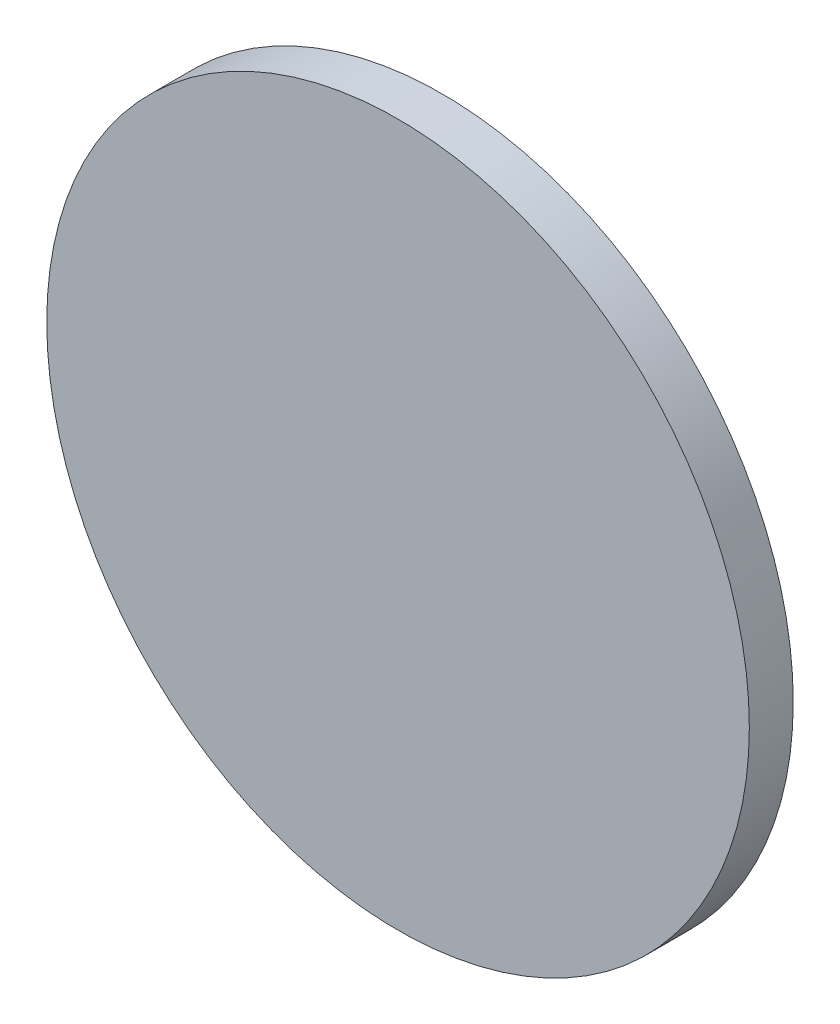
SolidWorks part; units mm, degrees
ref_plane "Front Plane" through (0, 0, 0) normal (0, 0, 1) x (1, 0, 0)
ref_plane "Top Plane" through (0, 0, 0) normal (0, 1, 0) x (1, 0, 0)
ref_plane "Right Plane" through (0, 0, 0) normal (1, 0, 0) x (0, 0, -1)
sketch "Sketch1" plane through (0, 0, 0) normal (0, 0, 1) x (1, 0, 0)
  circle A0 centre (0, 0) radius 8
  dimension "D1" = 16
extrude "Boss-Extrude1" add sketch "Sketch1" along normal blind 1
